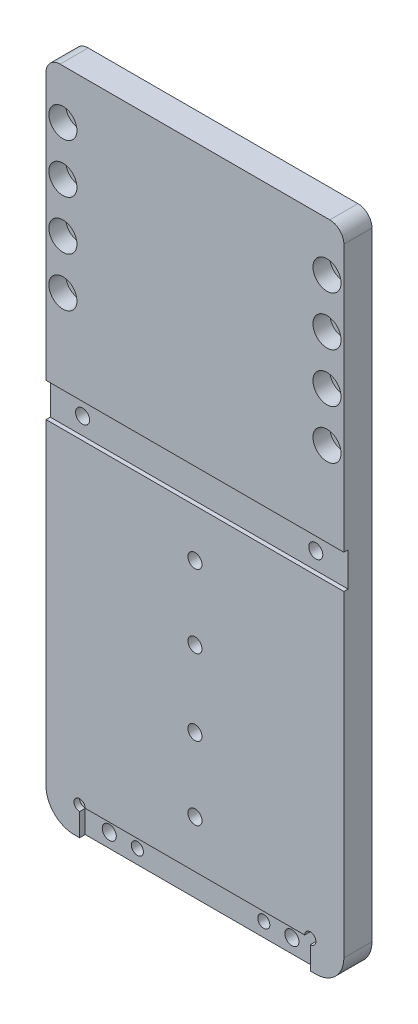
from build123d import *

# Parameters (mm, degrees)
SKETCH_1_W                = 80
SKETCH_1_H                = 235
EXTRUDE_1_DEPTH           = 10
SKETCH_20_W               = 82
SKETCH_20_H               = 14.219263271
CUT_EXTRUDE_3_DEPTH       = 2
HOLE_WIZARD_4_D           = 4.3
HOLE_WIZARD_4_CBORE_D     = 8
HOLE_WIZARD_4_CBORE_DEPTH = 5
SKETCH_26_W               = 13
SKETCH_26_H               = 87.5
EXTRUDE_3_DEPTH           = 10
FILLET_5_R                = 5
HOLE_WIZARD_1_D           = 5.4
HOLE_WIZARD_1_CBORE_D     = 10
HOLE_WIZARD_1_CBORE_DEPTH = 6
PATTERN_LINEAR_2_COUNT    = 2
PATTERN_LINEAR_2_PITCH    = 17.5
MOVE_FACE_1_BY            = 13
MOVE_FACE_1_2_BY          = 13
SKETCH_30_W               = 265.385639797
SKETCH_30_H               = 12.1
CUT_EXTRUDE_7_DEPTH       = 1.5
SKETCH_31_W               = 11.95
SKETCH_31_H               = 17.539728067
SKETCH_31_H_2             = 20.784895231
EXTRUDE_4_DEPTH           = 10
SKETCH_32_R               = 2
CUT_EXTRUDE_8_DEPTH       = 2
MM_1_D                    = 5
MM_1_DEPTH                = 10.1
MM_1_TIP                  = 1.502151548
FILLET_6_R                = 10
HOLE_WIZARD_M6_1_D        = 5
HOLE_WIZARD_M6_1_DEPTH    = 15
HOLE_WIZARD_M6_1_TIP      = 1.502151548
HOLE_WIZARD_M6_2_D        = 5
HOLE_WIZARD_M6_2_DEPTH    = 15
HOLE_WIZARD_M6_2_TIP      = 1.502151548
HOLE_WIZARD_M6_3_D        = 5
HOLE_WIZARD_M6_4_D        = 5


with BuildPart() as part:
    # 草图1 → 凸台-拉伸1 (new body)
    with BuildSketch(Plane.XY):
        with Locations((0, -117.5)):
            Rectangle(SKETCH_1_W, SKETCH_1_H)
    extrude(amount=EXTRUDE_1_DEPTH)

    # 草图20 → 切除-拉伸3 (cut)
    with BuildSketch(Plane.XY.offset(10)):
        with Locations((0, -232.009631635)):
            Rectangle(SKETCH_20_W, SKETCH_20_H)
    extrude(amount=-CUT_EXTRUDE_3_DEPTH, mode=Mode.SUBTRACT)

    # 打孔尺寸(%根据)开槽圆柱头螺钉的类型4 (through all)
    with Locations(Plane(origin=(0, 0, 0), x_dir=(-1, 0, 0), z_dir=(0, 0, -1))):
        with Locations((-22.5, -230), (22.5, -230)):
            CounterBoreHole(HOLE_WIZARD_4_D / 2, HOLE_WIZARD_4_CBORE_D / 2, HOLE_WIZARD_4_CBORE_DEPTH)

    # 草图26 → 凸台-拉伸3 (add)
    with BuildSketch(Plane.XY.offset(10)):
        with Locations((46.5, -43.75)):
            Rectangle(SKETCH_26_W, SKETCH_26_H)
    extrude_3 = extrude(amount=-EXTRUDE_3_DEPTH)

    # 镜向1: 凸台-拉伸3 across plane
    add(extrude_3.mirror(Plane(origin=(0, 0, 0), x_dir=(0, 0, 1), z_dir=(1, 0, 0))))

    # 圆角5
    fillet_5_edges = [part.edges().sort_by_distance(p)[0] for p in [
        (53, 0, 5),
        (-53, 0, 5),
    ]]
    fillet(fillet_5_edges, radius=FILLET_5_R)

    # 打孔尺寸(%根据)内六角圆柱头螺钉的类型1 (through all)
    with Locations(Plane.XY.offset(10)):
        with Locations((-47, -17.5), (-47, -52.5), (47, -52.5), (47, -17.5)):
            hole_wizard_1 = CounterBoreHole(HOLE_WIZARD_1_D / 2, HOLE_WIZARD_1_CBORE_D / 2, HOLE_WIZARD_1_CBORE_DEPTH)

    # 阵列(线性)2: 打孔尺寸(%根据)内六角圆柱头螺钉的类型1 ×2
    with Locations(*[(0, -i * PATTERN_LINEAR_2_PITCH, 0) for i in range(1, PATTERN_LINEAR_2_COUNT)]):
        add(hole_wizard_1, mode=Mode.SUBTRACT)

    # Move Face 1: a face moved outward by 13.0
    extrude(part.faces().sort_by_distance((40, -160.296095683, 4.94445972))[0], amount=MOVE_FACE_1_BY, dir=(1, 0, 0))

    # Move Face 1 2: a face moved outward by 13.0
    extrude(part.faces().sort_by_distance((-40, -160.296095683, 4.94445972))[0], amount=MOVE_FACE_1_2_BY, dir=(-1, 0, 0))

    # 草图30 → 切除-拉伸7 (cut)
    with BuildSketch(Plane.XY.offset(10)):
        with Locations((-68.564117246, -106)):
            Rectangle(SKETCH_30_W, SKETCH_30_H)
    extrude(amount=-CUT_EXTRUDE_7_DEPTH, mode=Mode.SUBTRACT)

    # 草图31 → 凸台-拉伸4 (add)
    with BuildSketch(Plane.XY.offset(10)):
        with Locations((-47.025, -226.230135967)):
            Rectangle(SKETCH_31_W, SKETCH_31_H)
        with Locations((47.025, -224.607552385)):
            Rectangle(SKETCH_31_W, SKETCH_31_H_2)
    extrude(amount=-EXTRUDE_4_DEPTH)

    # 草图32 → 切除-拉伸8 (cut)
    with BuildSketch(Plane.XY.offset(10)):
        with Locations((-41.05, -224.9)):
            Circle(SKETCH_32_R)
        with Locations((41.05, -224.9)):
            Circle(SKETCH_32_R)
    extrude(amount=-CUT_EXTRUDE_8_DEPTH, mode=Mode.SUBTRACT)

    # 大小mm 暗销孔1
    with Locations(Plane(origin=(0, 0, 0), x_dir=(-1, 0, 0), z_dir=(0, 0, -1))):
        with Locations((-32.5, -230), (32.5, -230)):
            Hole(MM_1_D / 2, depth=MM_1_DEPTH)
            with Locations((0, 0, -(MM_1_DEPTH + MM_1_TIP / 2))):  # 118° drill point
                Cone(0, MM_1_D / 2, MM_1_TIP, mode=Mode.SUBTRACT)

    # 圆角6
    fillet_6_edges = [part.edges().sort_by_distance(p)[0] for p in [
        (53, -235, 5),
        (-53, -235, 5),
    ]]
    fillet(fillet_6_edges, radius=FILLET_6_R)

    # M6 螺纹孔1
    with Locations(Plane.XY.offset(10)):
        with Locations((-41.5, -106), (41.5, -106)):
            Hole(HOLE_WIZARD_M6_1_D / 2, depth=HOLE_WIZARD_M6_1_DEPTH)
            with Locations((0, 0, -(HOLE_WIZARD_M6_1_DEPTH + HOLE_WIZARD_M6_1_TIP / 2))):  # 118° drill point
                Cone(0, HOLE_WIZARD_M6_1_D / 2, HOLE_WIZARD_M6_1_TIP, mode=Mode.SUBTRACT)

    # M6 螺纹孔2
    with Locations(Plane.XY.offset(10)):
        with Locations((0, -208)):
            Hole(HOLE_WIZARD_M6_2_D / 2, depth=HOLE_WIZARD_M6_2_DEPTH)
            with Locations((0, 0, -(HOLE_WIZARD_M6_2_DEPTH + HOLE_WIZARD_M6_2_TIP / 2))):  # 118° drill point
                Cone(0, HOLE_WIZARD_M6_2_D / 2, HOLE_WIZARD_M6_2_TIP, mode=Mode.SUBTRACT)

    # M6 螺纹孔3 (through all)
    with Locations(Plane.XY.offset(10)):
        with Locations((0, -155), (0, -182)):
            Hole(HOLE_WIZARD_M6_3_D / 2)

    # M6 螺纹孔4 (through all)
    with Locations(Plane.XY.offset(10)):
        with Locations((0, -129)):
            Hole(HOLE_WIZARD_M6_4_D / 2)


solid = part.part
